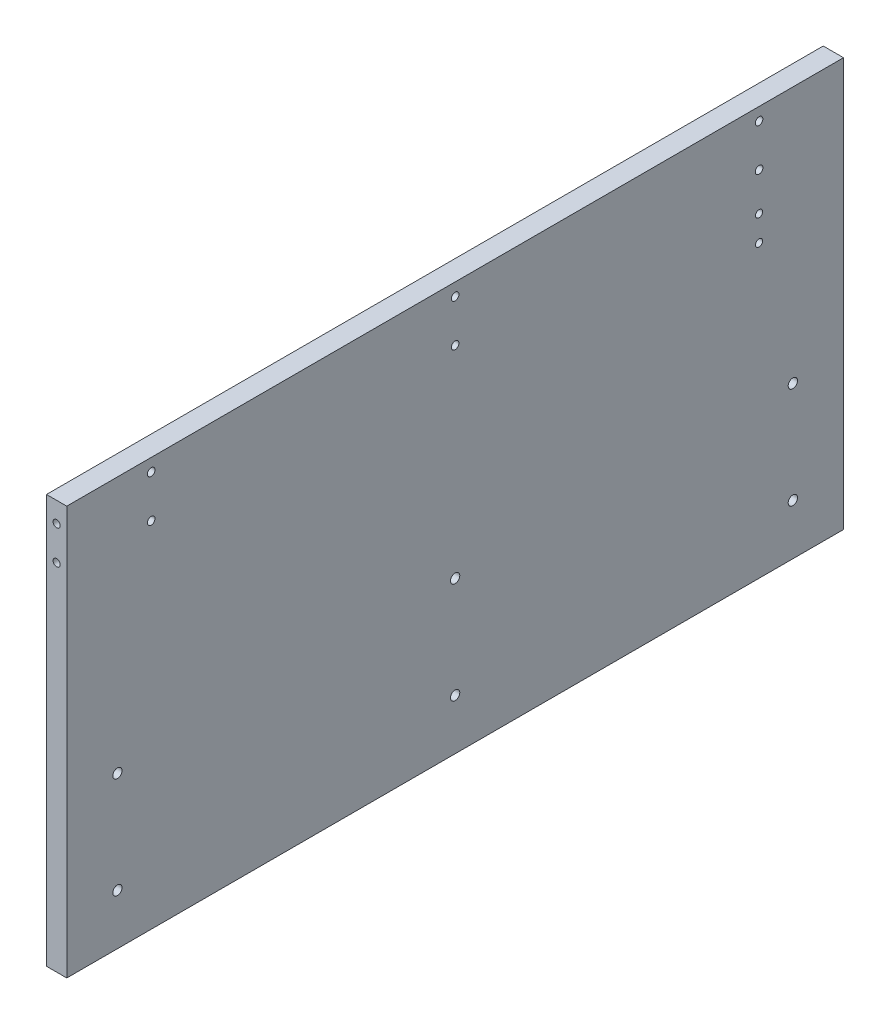
SolidWorks part; units mm, degrees
material "6061 合金"
ref_plane "前视基准面" through (0, 0, 0) normal (0, 0, 1) x (1, 0, 0)
ref_plane "上视基准面" through (0, 0, 0) normal (0, 1, 0) x (1, 0, 0)
ref_plane "右视基准面" through (0, 0, 0) normal (1, 0, 0) x (0, 0, -1)
sketch "草图1" plane through (0, 0, 0) normal (0, 0, 1) x (1, 0, 0)
  line L1 (-6, 121) -> (6, 121)
  line L2 (-6, 121) -> (-6, -121)
  line L3 (-6, -121) -> (6, -121)
  line L4 (6, 121) -> (6, -121)
  line L5 (-6, 121) -> (6, -121) construction
  line L6 (-6, -121) -> (6, 121) construction
  point P0 (0, 0)
  dimension "D1" = 12
  dimension "D2" = 242
extrude "凸台-拉伸1" add sketch "草图1" along normal mid plane 460
hole_wizard "M5 螺纹孔1" positions "草图3" profile "草图2" tap size "M5" standard "GB"
sketch "草图3" plane through (0, -121, 0) normal (0, -1, 0) x (1, 0, 0)
  point P0 (0, 200)
  point P4 (0, 0)
  point P6 (0, -200)
  dimension "D1" = 200
  dimension "D3" = 200
sketch "草图2" plane through (0, -121, 200) normal (1, 0, 0) x (0, 0, -1)
  line L0 (0, 0) -> (0, 15.2618)
  line L1 (0, 15.2618) -> (2.1, 14)
  line L2 (2.1, 14) -> (2.1, 0)
  line L5 (2.1, 0) -> (0, 0)
  line L10 (0, 15.2618) -> (-2.1, 14) construction
  line L11 (0, -6.35) -> (0, 107.95) construction
  dimension "螺纹孔钻头直径" = 4.2
  dimension "螺纹孔钻头深度" = 14
  dimension "导头角度" = 118
cosmetic thread "孔螺蚊线1"
cosmetic thread "孔螺蚊线2"
cosmetic thread "孔螺蚊线4"
hole_wizard "打孔尺寸(%根据)内六角圆柱头螺钉的类型1" positions "草图5" profile "草图4" counterbore size "M5" standard "GB"
sketch "草图5" plane through (-6, 0, 0) normal (-1, 0, 0) x (0, 0, 1)
  line L0 (230, -121) -> (-230, -121) construction
  line L1 (230, 121) -> (230, -121) construction
  point P0 (200, -31)
  point P2 (200, -91)
  point P19 (0, -31)
  point P20 (0, -91)
  point P21 (-200, -31)
  point P22 (-200, -91)
  dimension "D1" = 60
  dimension "D2" = 30
  dimension "D3" = 30
  dimension "D4" = 3
sketch "草图4" plane through (-6, -31, 200) normal (0, 1, 0) x (0, 0, 1)
  line L0 (0, 0) -> (0, 15.6524)
  line L1 (0, 15.6524) -> (2.75, 14)
  line L2 (2.75, 14) -> (2.75, 5.7)
  line L3 (2.75, 5.7) -> (5, 5.7)
  line L4 (5, 5.7) -> (5, 0)
  line L5 (5, 0) -> (0, 0)
  line L10 (0, 15.6524) -> (-2.75, 14) construction
  line L11 (0, -6.35) -> (0, 107.95) construction
  dimension "孔直径" = 5.5
  dimension "孔深度" = 14
  dimension "柱形沉头孔直径" = 10
  dimension "柱形沉头孔深度" = 5.7
  dimension "导头角度" = 118
hole_wizard "打孔尺寸(%根据)内六角圆柱头螺钉的类型2" positions "草图7" profile "草图6" counterbore size "M4" standard "GB"
sketch "草图7" plane through (-6, 0, 0) normal (1, 0, 0) x (0, 0, -1)
  line L0 (-230, 121) -> (230, 121) construction
  line L1 (230, -121) -> (230, 121) construction
  point P0 (180, 113.5)
  point P2 (180, 88.5)
  point P14 (0, 113.5)
  point P15 (0, 88.5)
  point P16 (-180, 113.5)
  point P17 (-180, 88.5)
  dimension "D1" = 25
  dimension "D2" = 7.5
  dimension "D3" = 50
  dimension "D4" = 3
sketch "草图6" plane through (-6, 113.5, -180) normal (0, 1, 0) x (0, 0, 1)
  line L0 (0, 0) -> (0, 15.3519)
  line L1 (0, 15.3519) -> (2.25, 14)
  line L2 (2.25, 14) -> (2.25, 4.6)
  line L3 (2.25, 4.6) -> (4, 4.6)
  line L4 (4, 4.6) -> (4, 0)
  line L5 (4, 0) -> (0, 0)
  line L10 (0, 15.3519) -> (-2.25, 14) construction
  line L11 (0, -6.35) -> (0, 107.95) construction
  dimension "孔直径" = 4.5
  dimension "孔深度" = 14
  dimension "柱形沉头孔直径" = 8
  dimension "柱形沉头孔深度" = 4.6
  dimension "导头角度" = 118
hole_wizard "M5 螺纹孔2" positions "草图9" profile "草图8" tap size "M5" standard "GB"
sketch "草图9" plane through (0, 0, -230) normal (0, 0, -1) x (-1, 0, 0)
  line L0 (-6, 121) -> (6, 121) construction
  line L1 (6, 121) -> (6, -121) construction
  point P0 (0, 109)
  point P2 (0, 89)
  dimension "D1" = 20
  dimension "D2" = 12
  dimension "D3" = 6
sketch "草图8" plane through (0, 109, -230) normal (1, 0, 0) x (0, 1, 0)
  line L0 (0, 0) -> (0, 15.2618)
  line L1 (0, 15.2618) -> (2.1, 14)
  line L2 (2.1, 14) -> (2.1, 0)
  line L5 (2.1, 0) -> (0, 0)
  line L10 (0, 15.2618) -> (-2.1, 14) construction
  line L11 (0, -6.35) -> (0, 107.95) construction
  dimension "螺纹孔钻头直径" = 4.2
  dimension "螺纹孔钻头深度" = 14
  dimension "导头角度" = 118
cosmetic thread "孔螺蚊线5"
cosmetic thread "孔螺蚊线6"
mirror "镜向1" about plane through (0, 0, 0) normal (0, 0, 1) of "M5 螺纹孔2"
hole_wizard "M5 螺纹孔3" positions "草图11" profile "草图10" tap size "M5" standard "GB"
sketch "草图11" plane through (6, 0, 0) normal (1, 0, 0) x (0, 0, -1)
  line L0 (-230, 121) -> (230, 121) construction
  line L1 (230, -121) -> (230, 121) construction
  point P0 (180, 66)
  point P2 (180, 51)
  dimension "D1" = 55
  dimension "D2" = 15
  dimension "D3" = 50
sketch "草图10" plane through (6, 66, -180) normal (0, 1, 0) x (0, 0, -1)
  line L0 (0, 0) -> (0, 15.2618)
  line L1 (0, 15.2618) -> (2.1, 14)
  line L2 (2.1, 14) -> (2.1, 0)
  line L5 (2.1, 0) -> (0, 0)
  line L10 (0, 15.2618) -> (-2.1, 14) construction
  line L11 (0, -6.35) -> (0, 107.95) construction
  dimension "螺纹孔钻头直径" = 4.2
  dimension "螺纹孔钻头深度" = 14
  dimension "导头角度" = 118
cosmetic thread "孔螺蚊线7"
cosmetic thread "孔螺蚊线8"
